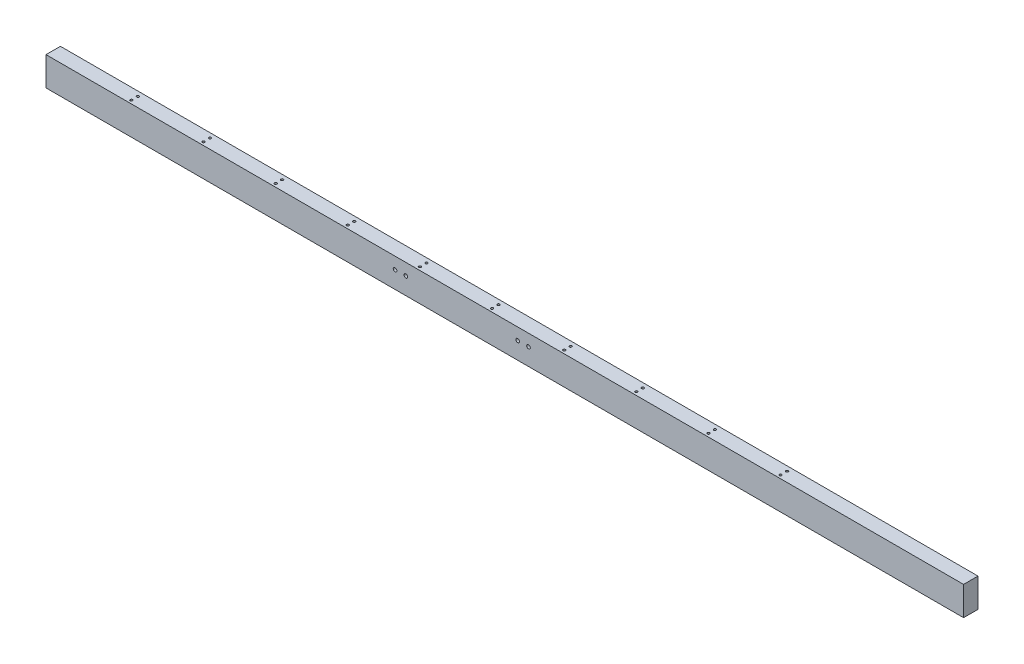
from build123d import *

# Parameters (mm, degrees)
SKETCH_1_W             = 2544
SKETCH_1_H             = 80
EXTRUDE_1_DEPTH        = 40
SKETCH_2_R             = 3.335467959
SKETCH_2_R_2           = 3.3
CUT_EXTRUDE_1_DEPTH    = 40
PATTERN_LINEAR_1_COUNT = 10
PATTERN_LINEAR_1_PITCH = 200
SKETCH_3_R             = 4.5
CUT_EXTRUDE_2_DEPTH    = 40
SKETCH_4_R             = 5
CUT_EXTRUDE_3_DEPTH    = 20
SKETCH_5_R             = 7.5
CUT_EXTRUDE_4_DEPTH    = 15


with BuildPart() as part:
    # 草图1 → 凸台-拉伸1 (new body)
    with BuildSketch(Plane.XY):
        with Locations((1272, -40)):
            Rectangle(SKETCH_1_W, SKETCH_1_H)
    extrude(amount=EXTRUDE_1_DEPTH)

    # 草图2 → 切除-拉伸1 (cut)
    with BuildSketch(Plane(origin=(0, 0, 0), x_dir=(1, 0, 0), z_dir=(0, 1, 0))):
        with Locations(Location((227.728390154, -13, 0), (0, 0, 270))):
            Circle(SKETCH_2_R)
        with Locations(Location((227.728390154, -31, 0), (0, 0, 270))):
            Circle(SKETCH_2_R_2)
    cut_extrude_1 = extrude(amount=-CUT_EXTRUDE_1_DEPTH, mode=Mode.SUBTRACT)

    # 阵列(线性)1: 切除-拉伸1 ×10
    with Locations(*[(i * PATTERN_LINEAR_1_PITCH, 0, 0) for i in range(1, PATTERN_LINEAR_1_COUNT)]):
        add(cut_extrude_1, mode=Mode.SUBTRACT)

    # 草图3 → 切除-拉伸2 (cut)
    with BuildSketch(Plane.XZ.offset(80)):
        with Locations(Location((458, 23.1, 0), (0, 0, 270))):
            Circle(SKETCH_3_R)
        with Locations(Location((581, 23.1, 0), (0, 0, 270))):
            Circle(SKETCH_3_R)
        with Locations(Location((1958, 23.1, 0), (0, 0, 270))):
            Circle(SKETCH_3_R)
        with Locations(Location((2081, 23.1, 0), (0, 0, 270))):
            Circle(SKETCH_3_R)
    extrude(amount=-CUT_EXTRUDE_2_DEPTH, mode=Mode.SUBTRACT)

    # 草图4 → 切除-拉伸3 (cut)
    with BuildSketch(Plane.XY.offset(40)):
        with Locations((1337.7370976, -32.684091126)):
            Circle(SKETCH_4_R)
        with Locations((1307.7370976, -32.684091126)):
            Circle(SKETCH_4_R)
        with Locations((997.7370976, -32.684091126)):
            Circle(SKETCH_4_R)
        with Locations((967.7370976, -32.684091126)):
            Circle(SKETCH_4_R)
    extrude(amount=-CUT_EXTRUDE_3_DEPTH, mode=Mode.SUBTRACT)

    # 草图5 → 切除-拉伸4 (cut)
    with BuildSketch(Plane(origin=(0, 0, 0), x_dir=(-1, 0, 0), z_dir=(0, 0, -1))):
        with Locations((-1265.2370976, -26)):
            Circle(SKETCH_5_R)
        with Locations((-1040.2370976, -26)):
            Circle(SKETCH_5_R)
    extrude(amount=-CUT_EXTRUDE_4_DEPTH, mode=Mode.SUBTRACT)


solid = part.part
